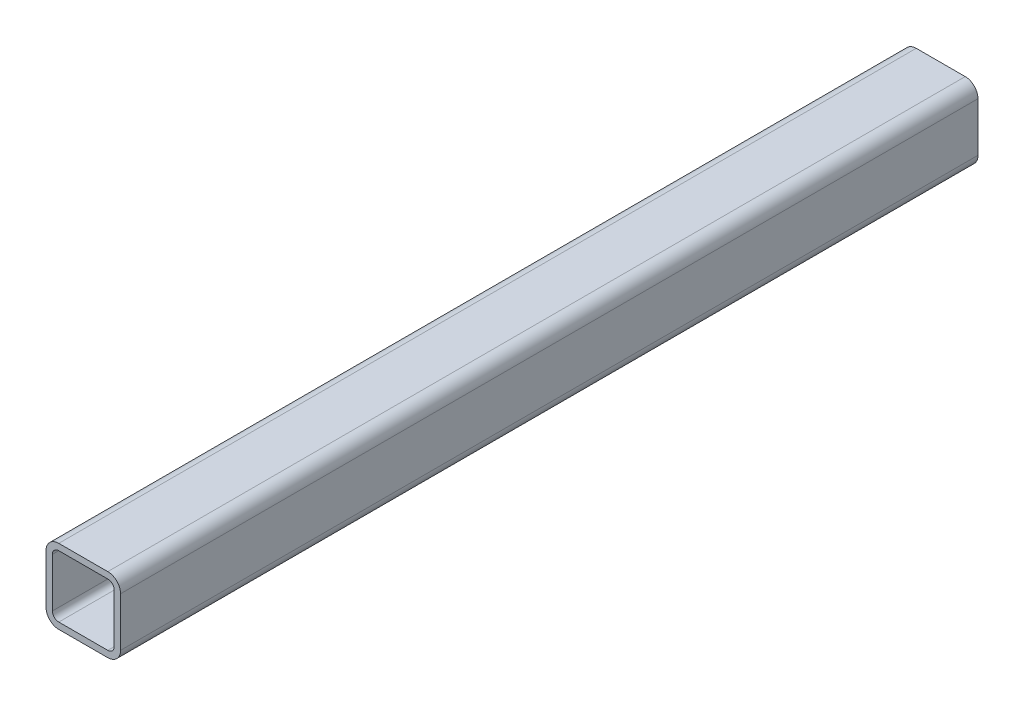
from build123d import *

# Parameters (mm, degrees)
BOSS_EXTRUDE1_DEPTH = 805


with BuildPart() as part:
    # Sketch1 → Boss-Extrude1 (new body)
    with BuildSketch(Plane.XY):
        with BuildLine():
            Line((12, 0), (58, 0))
            ThreePointArc((58, 0), (66.485281374, 3.514718626), (70, 12))
            Line((70, 12), (70, 58))
            ThreePointArc((70, 58), (66.485281374, 66.485281374), (58, 70))
            Line((58, 70), (12, 70))
            ThreePointArc((12, 70), (3.514718626, 66.485281374), (0, 58))
            Line((0, 58), (0, 12))
            ThreePointArc((0, 12), (3.514718626, 3.514718626), (12, 0))
        make_face()
        with BuildLine():
            Line((12, 6), (58, 6))
            ThreePointArc((58, 6), (62.242640687, 7.757359313), (64, 12))
            Line((64, 12), (64, 58))
            ThreePointArc((64, 58), (62.242640687, 62.242640687), (58, 64))
            Line((58, 64), (12, 64))
            ThreePointArc((12, 64), (7.757359313, 62.242640687), (6, 58))
            Line((6, 58), (6, 12))
            ThreePointArc((6, 12), (7.757359313, 7.757359313), (12, 6))
        make_face(mode=Mode.SUBTRACT)
    extrude(amount=BOSS_EXTRUDE1_DEPTH)


solid = part.part
